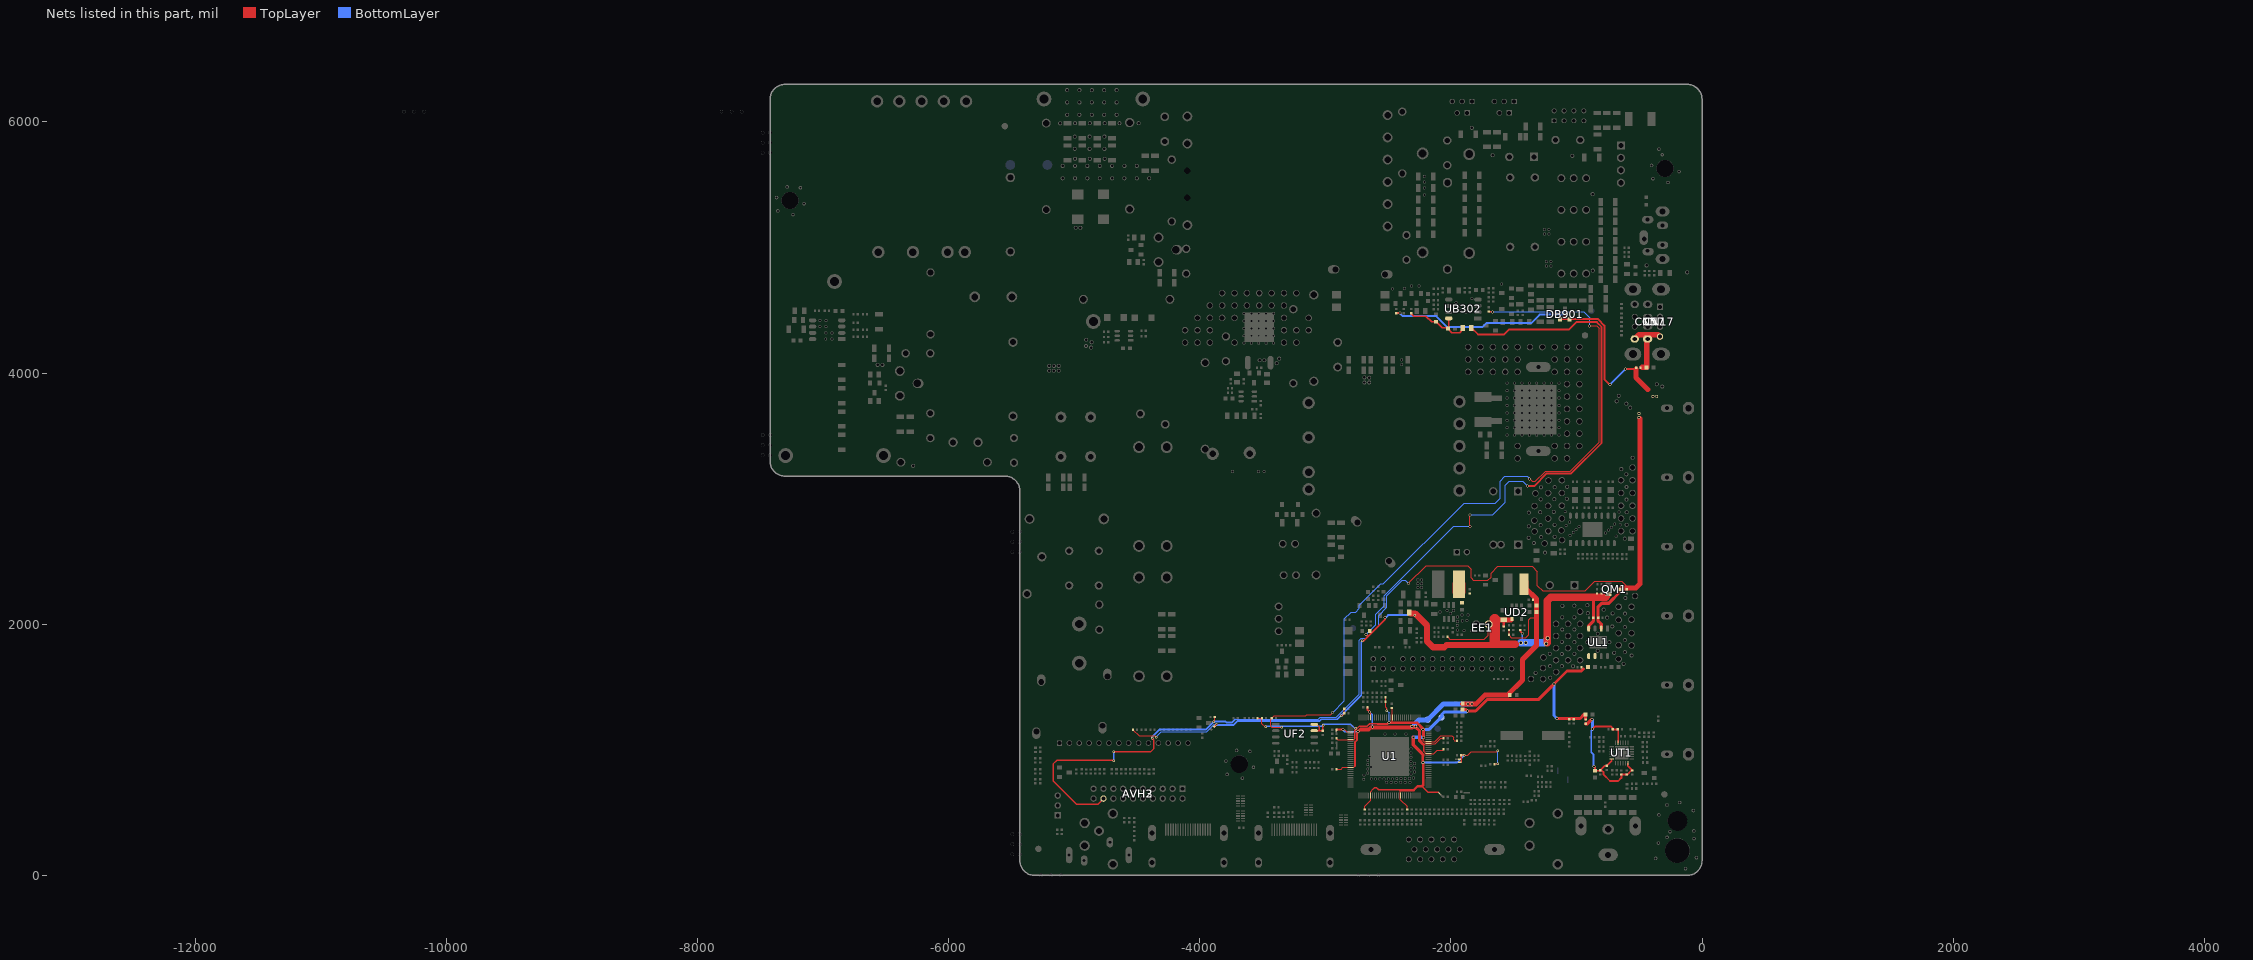
[diagram p0: the nets of this part, all layers, seen from the top]
# Altium PCB MISC84277.PcbDoc (part 6 of 15)
Units mil, origin at the board's own origin, x right, y up, seen from the top; angles counter-clockwise.
Board outline 7422.08 x 6299.21 mil, 2 copper layers (TopLayer, BottomLayer), stack 61.855 mil thick; 709 components, 395 nets, 2812 pads, 811 vias.

## Free pads (board coordinates)
  oval 196.85x157.48 on Keep-Out: 0(-12538.98,6102.21) 0(-375.96,-19.69)
  round 78.74 on Keep-Out: 0(-12170.24,6219.32) 0(-8343.94,6219.32) 0(-4571,-136.8) 0(-744.7,-136.8)
  round 27.56 hole 27.56 unplated: 0(-10337.93,6082.52) 0(-10257.61,6082.52) 0(-10177.3,6082.52) 0(-7809.45,6082.52) 0(-7729.14,6082.52) 0(-7648.82,6082.52) 0(-7481.5,3346.46) 0(-7481.5,3426.77) 0(-7481.5,3507.09) 0(-7481.5,5754.57) 0(-7481.5,5834.89) 0(-7481.5,5915.2) 0(-7422.44,3346.46) 0(-7422.44,3426.77) 0(-7422.44,3507.09) 0(-7422.44,5754.57) 0(-7422.44,5834.89) 0(-7422.44,5915.2) 0(-5492.5,167.48) 0(-5492.5,247.79) 0(-5492.5,328.11) 0(-5492.5,2575.59) 0(-5492.5,2655.9) 0(-5492.5,2736.22) 0(-5433.44,167.48) 0(-5433.44,247.79) 0(-5433.44,328.11) 0(-5433.44,2575.59) 0(-5433.44,2655.9) 0(-5433.44,2736.22) 0(-5266.12,0) 0(-5185.8,0) 0(-5105.49,0) 0(-2737.64,0) 0(-2657.33,0) 0(-2577.01,0)
  round 137.8 on Keep-Out: 0(-5312.1,562.78) 0(-196.85,5708.82)
  round 157.48 on Keep-Out: 0(-197.22,6102.36)
  oval 157.48x196.85 on Keep-Out: 0(-196.85,3503.94)
  round 23.62 hole 15.75 paste-15.75 mask-15.75: VIA5(-7026.5,4370.37) VIA5(-7025.59,4419.29) VIA5(-6979.39,4271.61) VIA5(-6978.49,4320.53) VIA5(-6977.58,4369.46) VIA5(-6976.67,4418.38) VIA5(-6930.47,4270.7) VIA5(-6929.56,4319.62) VIA5(-3740.16,3216.09) VIA5(-3648.83,4297.38) VIA5(-3648.83,4356.44) VIA5(-3648.83,4415.49) VIA5(-3648.83,4474.55) VIA5(-3648.83,4238.33) VIA5(-3589.77,4238.33) VIA5(-3589.77,4297.38) VIA5(-3589.77,4356.44) VIA5(-3589.77,4415.49) VIA5(-3589.77,4474.55) VIA5(-3533.46,3216.09) VIA5(-3530.72,4297.38) VIA5(-3530.72,4474.55) VIA5(-3530.72,4238.33) VIA5(-3530.72,4356.44) VIA5(-3530.72,4415.49) VIA5(-3488.19,3216.54) VIA5(-3471.66,4238.33) VIA5(-3471.66,4297.38) VIA5(-3471.66,4356.44) VIA5(-3471.66,4415.49) VIA5(-3471.66,4474.55) VIA5(-3412.61,4238.33) VIA5(-3412.61,4297.38) VIA5(-3412.61,4356.44) VIA5(-3412.61,4415.49) VIA5(-3412.61,4474.55) VIA5(-2694.55,765.25) VIA5(-2693.4,797.4) VIA5(-2662.7,814) VIA5(-2662.7,847.8) VIA5(-2662.7,881.6) VIA5(-2662.7,915.4) VIA5(-2648.2,948.3) VIA5(-2635.5,864.3) VIA5(-2634.5,769.2) VIA5(-2600.7,769.2) VIA5(-2566.9,769.2) VIA5(-2533.1,769.2) VIA5(-2525.21,1124.32) VIA5(-2513.2,741) VIA5(-2499.3,769.2) VIA5(-2476,741) VIA5(-2466.54,4671.26) VIA5(-2465.5,769.2) VIA5(-2445,1124) VIA5(-2438.8,741) VIA5(-2431.7,770.9) VIA5(-2401.6,741) VIA5(-2397.9,770.9) VIA5(-2392.66,4067.75) VIA5(-2392.66,4105.75) VIA5(-2370.87,4674) VIA5(-2364.4,741) VIA5(-2364.1,770.9) VIA5(-2358.3,1124.32) VIA5(-2330.3,770.9) VIA5(-2327.2,741) VIA5(-2319.2,805.4) VIA5(-2319.2,839.2) VIA5(-2319.2,873) VIA5(-2319.2,906.8) VIA5(-2319.2,940.6) VIA5(-2319.2,974.4) VIA5(-2319.2,1008.2) VIA5(-2314.96,4693.81) VIA5(-2312.19,1186.7) VIA5(-2297.6,775.2) VIA5(-2290.9,823) VIA5(-2290.9,856.8) VIA5(-2290.9,890.6) VIA5(-2281.65,1186.7) VIA5(-2264.25,2293.31) VIA5(-2264.25,2323.31) VIA5(-2264.25,2353.31) VIA5(-2253.94,4693.81) VIA5(-2234.25,2293.31) VIA5(-2234.25,2323.31) VIA5(-2234.25,2353.31) VIA5(-2221.6,898.2) VIA5(-2212.6,5419.29) VIA5(-2212.6,5474.41) VIA5(-2212.6,5521.65) VIA5(-2212.6,5566.93) VIA5(-2087.7,2097.06) VIA5(-2030,2110) VIA5(-2002,2087) VIA5(-1980,2109) VIA5(-1958.5,4561.5) VIA5(-1950,1991) VIA5(-1948.82,1952.76) VIA5(-1948,2022) VIA5(-1948,2058) VIA5(-1929.13,4535.43) VIA5(-1923,4495.5) VIA5(-1912,2074) VIA5(-1910,2027) VIA5(-1895.67,1948.82) VIA5(-1879.92,4487.1) VIA5(-1874,2030) VIA5(-1866,1366) VIA5(-1863,2074) VIA5(-1836.61,1948.82) VIA5(-1834,1366) VIA5(-1832.68,4592.52) VIA5(-1596,4709) VIA5(-1552.98,3506) VIA5(-1552.98,3565.05) VIA5(-1552.98,3624.11) VIA5(-1552.98,3683.16) VIA5(-1552.98,3742.22) VIA5(-1552.98,3801.27) VIA5(-1552.98,3860.33) VIA5(-1552.98,3919.38) VIA5(-1493.92,3506) VIA5(-1493.92,3565.05) VIA5(-1493.92,3624.11) VIA5(-1493.92,3683.16) VIA5(-1493.92,3742.22) VIA5(-1493.92,3801.27) VIA5(-1493.92,3860.33) VIA5(-1493.92,3919.38) VIA5(-1434.87,3506) VIA5(-1434.87,3565.05) VIA5(-1434.87,3624.11) VIA5(-1434.87,3683.16) VIA5(-1434.87,3742.22) VIA5(-1434.87,3801.27) VIA5(-1434.87,3860.33) VIA5(-1434.87,3919.38) VIA5(-1375.81,3506) VIA5(-1375.81,3565.05) VIA5(-1375.81,3624.11) VIA5(-1375.81,3683.16) VIA5(-1375.81,3742.22) VIA5(-1375.81,3801.27) VIA5(-1375.81,3860.33) VIA5(-1375.81,3919.38) VIA5(-1316.76,3742.22) VIA5(-1316.76,3860.33) VIA5(-1316.76,3506) VIA5(-1316.76,3565.05) VIA5(-1316.76,3624.11) VIA5(-1316.76,3683.16) VIA5(-1316.76,3801.27) VIA5(-1316.76,3919.38) VIA5(-1257.7,3565.05) VIA5(-1257.7,3683.16) VIA5(-1257.7,3742.22) VIA5(-1257.7,3801.27) VIA5(-1257.7,3860.33) VIA5(-1257.7,3919.38) VIA5(-1257.7,3506) VIA5(-1257.7,3624.11) VIA5(-1255.91,5108.27) VIA5(-1255.91,5143.7) VIA5(-1240.16,4852.36) VIA5(-1240.16,4887.8) VIA5(-1220.47,5108.27) VIA5(-1220.47,5143.7) VIA5(-1204.72,4852.36) VIA5(-1204.72,4887.8) VIA5(-1198.65,3506) VIA5(-1198.65,3565.05) VIA5(-1198.65,3624.11) VIA5(-1198.65,3683.16) VIA5(-1198.65,3742.22) VIA5(-1198.65,3801.27) VIA5(-1198.65,3860.33) VIA5(-1198.65,3919.38) VIA5(-1139.59,3506) VIA5(-1139.59,3565.05) VIA5(-1139.59,3624.11) VIA5(-1139.59,3683.16) VIA5(-1139.59,3742.22) VIA5(-1139.59,3801.27) VIA5(-1139.59,3860.33) VIA5(-1139.59,3919.38) VIA5(-1090,2896) VIA5(-1082,2786) VIA5(-1054.5,2812.85) VIA5(-1051,2708) VIA5(-1026,2732) VIA5(-1003,2755) VIA5(-979,2778) VIA5(-770,2726) VIA5(-746,2749) VIA5(-722,2772) VIA5(-696,2798) VIA5(-684,2701) VIA5(-660,2894) VIA5(-652,2792) VIA5(-503,3648) VIA5(-503,3678) VIA5(-391.95,3813.95) VIA5(-361.95,3813.95)
  round 31.5 hole 19.68 paste-15.75 mask-15.75: VIA5(-6566,4065) VIA5(-6528,4065) VIA5(-6283.46,3261.81) VIA5(-5200,4018.9) VIA5(-5200,4056.9) VIA5(-5162,4018.9) VIA5(-5162,4056.9) VIA5(-5124,4018.9) VIA5(-5124,4056.9) VIA5(-5112.75,5989.43) VIA5(-5092.52,5551.18) VIA5(-5092.52,5649.61) VIA5(-5057.09,6057.09) VIA5(-5057.09,6155.51) VIA5(-5057.09,6253.94) VIA5(-4996.06,5785.43) VIA5(-4996.06,5883.86) VIA5(-4994.09,5551.18) VIA5(-4994.09,5649.61) VIA5(-4994.09,5706.69) VIA5(-4994.09,5990.16) VIA5(-4988.79,5157.48) VIA5(-4958.66,6057.09) VIA5(-4958.66,6155.51) VIA5(-4958.66,6253.94) VIA5(-4950.79,5157.48) VIA5(-4906.5,4215.9) VIA5(-4905.8,4265.5) VIA5(-4895.67,5551.18) VIA5(-4895.67,5649.61) VIA5(-4877.95,5785.43) VIA5(-4877.95,5883.86) VIA5(-4875.98,5706.69) VIA5(-4875.98,5990.16) VIA5(-4866.6,4203.6) VIA5(-4862.5,4245.5) VIA5(-4860.24,6057.09) VIA5(-4860.24,6155.51) VIA5(-4860.24,6253.94) VIA5(-4797.24,5551.18) VIA5(-4797.24,5649.61) VIA5(-4761.81,6057.09) VIA5(-4761.81,6155.51) VIA5(-4761.81,6253.94) VIA5(-4759.84,5785.43) VIA5(-4759.84,5883.86) VIA5(-4757.87,5990.16) VIA5(-4757.87,5706.69) VIA5(-4698.82,5551.18) VIA5(-4698.82,5649.61) VIA5(-4663.39,6057.09) VIA5(-4663.39,6155.51) VIA5(-4663.39,6253.94) VIA5(-4639.76,5990.16) VIA5(-4600.39,5551.18) VIA5(-4600.39,5649.61) VIA5(-4501.97,5551.18) VIA5(-4501.97,5649.61) VIA5(-4488.19,5990.16) VIA5(-4403.54,5551.18) VIA5(-3524.22,4102.36) VIA5(-3486.22,4102.36) VIA5(-3387.8,4078.74) VIA5(-3368.11,4116.14) VIA5(-2689.57,3925.2) VIA5(-2689.57,3965.17) VIA5(-2651.57,3925.2) VIA5(-2651.57,3963.2) VIA5(-1833.15,5953.3) VIA5(-1668.9,5735.1) VIA5(-1442.5,1851.35) VIA5(-1404.5,1851.35) VIA5(-1381,2687) VIA5(-1380,2780) VIA5(-1379.3,2889) VIA5(-1339,2647) VIA5(-1326,1612) VIA5(-1290,2892.6) VIA5(-1286,2790) VIA5(-1286,2994.6) VIA5(-1283,3090.6) VIA5(-1282,2694) VIA5(-1251,2571) VIA5(-1243,1845) VIA5(-1231,1888) VIA5(-1213,1764) VIA5(-1211,1667) VIA5(-1210,1574) VIA5(-1181,2894) VIA5(-1177,2996) VIA5(-1175,2696) VIA5(-1175,2791) VIA5(-1174,3092) VIA5(-1116,1667) VIA5(-1116,1763) VIA5(-1116,1859) VIA5(-1114,1958) VIA5(-1114,2054.64) VIA5(-1112.2,2145.67) VIA5(-1077,2999) VIA5(-1075,3094) VIA5(-1033.45,5730.08) VIA5(-1028,1665) VIA5(-1017.72,2147.64) VIA5(-1017,1764) VIA5(-1017,1858) VIA5(-1017,1958) VIA5(-1017,2054.64) VIA5(-914.5,1857.5) VIA5(-913.39,2151.57) VIA5(-910,2089) VIA5(-872.05,5425.2) VIA5(-870.08,4816.93) VIA5(-831.5,1788.5) VIA5(-831,1924.5) VIA5(-784,2116) VIA5(-757,2053) VIA5(-738.5,1857) VIA5(-715,1982) VIA5(-713,2086) VIA5(-701,1772) VIA5(-680.5,3775.28) VIA5(-663.82,3818.81) VIA5(-643,3236) VIA5(-625,1684) VIA5(-616,2682) VIA5(-615,1778) VIA5(-615,1874) VIA5(-615,1977) VIA5(-614,2085) VIA5(-611,2209) VIA5(-603,3194) VIA5(-602.2,3756.25) VIA5(-602,2993) VIA5(-602,3093) VIA5(-601,2792) VIA5(-601,2892) VIA5(-572.38,3725.25) VIA5(-562,1751) VIA5(-554,3326) VIA5(-442.4,4857.1) VIA5(-360.13,3911) VIA5(-317.13,3893.19) VIA5(-119,4802)
  round 51.18 hole 39.37 paste-15.75 mask-15.75: VIA5(-4117.27,4243.02) VIA5(-4117.27,4341.45) VIA5(-4018.84,4243.02) VIA5(-4018.84,4341.45) VIA5(-4018.84,4439.88) VIA5(-3920.42,4243.02) VIA5(-3920.42,4341.45) VIA5(-3920.42,4439.87) VIA5(-3920.42,4538.3) VIA5(-3821.99,4439.87) VIA5(-3821.99,4538.3) VIA5(-3821.99,4636.72) VIA5(-3723.57,4243.02) VIA5(-3723.57,4439.87) VIA5(-3723.57,4538.3) VIA5(-3723.57,4636.72) VIA5(-3625.14,4538.3) VIA5(-3625.14,4636.72) VIA5(-3526.72,4538.3) VIA5(-3526.72,4636.72) VIA5(-3428.29,4538.3) VIA5(-3428.29,4636.72) VIA5(-3329.87,4243.02) VIA5(-3329.87,4341.45) VIA5(-3329.87,4439.87) VIA5(-3329.87,4538.3) VIA5(-3329.86,4636.72) VIA5(-3231.44,4243.02) VIA5(-3231.44,4341.45) VIA5(-3231.44,4636.72) VIA5(-3133.02,4341.45) VIA5(-3133.02,4439.87) VIA5(-1862.93,4108.4) VIA5(-1862.93,4206.83) VIA5(-1862.93,4009.98) VIA5(-1764.51,4108.4) VIA5(-1764.51,4206.83) VIA5(-1764.51,4009.98) VIA5(-1666.08,4108.4) VIA5(-1666.08,4206.83) VIA5(-1666.08,4009.98) VIA5(-1567.66,4108.4) VIA5(-1567.66,4206.83) VIA5(-1567.66,4009.98) VIA5(-1469.23,3321) VIA5(-1469.23,4108.4) VIA5(-1469.23,4206.83) VIA5(-1469.23,3419.43) VIA5(-1469.23,4009.98) VIA5(-1370.81,4206.83) VIA5(-1363,1564) VIA5(-1336,2825) VIA5(-1335,2941) VIA5(-1334,2740) VIA5(-1327.5,3042.5) VIA5(-1272.38,4206.83) VIA5(-1267,1651) VIA5(-1266,1563) VIA5(-1264,1736) VIA5(-1254,2644) VIA5(-1226,2841) VIA5(-1226,2942.4) VIA5(-1226,3043.8) VIA5(-1225,2741) VIA5(-1223.2,3145.2) VIA5(-1173.96,3321) VIA5(-1173.96,4108.4) VIA5(-1173.96,4206.83) VIA5(-1173.96,3419.43) VIA5(-1173.96,4009.98) VIA5(-1163,1713.07) VIA5(-1163,1809.72) VIA5(-1163,1906.36) VIA5(-1163,2003) VIA5(-1162,1619) VIA5(-1121,2747) VIA5(-1117,2842.4) VIA5(-1117,2943.8) VIA5(-1117,3045.2) VIA5(-1117,3146.6) VIA5(-1115,2670) VIA5(-1075.53,3321) VIA5(-1075.53,4108.4) VIA5(-1075.53,4206.83) VIA5(-1075.53,3419.43) VIA5(-1075.53,3517.85) VIA5(-1075.53,3616.28) VIA5(-1075.53,3714.7) VIA5(-1075.53,3813.13) VIA5(-1075.53,3911.55) VIA5(-1075.53,4009.98) VIA5(-1067.25,1713.07) VIA5(-1067.25,1809.72) VIA5(-1067.25,1906.36) VIA5(-1067.25,2003) VIA5(-977.11,3419.43) VIA5(-977.11,3517.85) VIA5(-977.11,3616.28) VIA5(-977.11,3714.7) VIA5(-977.11,3813.13) VIA5(-977.11,3911.55) VIA5(-977.11,4009.98) VIA5(-977.11,4108.4) VIA5(-977.11,4206.83) VIA5(-971.5,1713.07) VIA5(-971.5,1809.72) VIA5(-971.5,1906.36) VIA5(-971.5,2003) VIA5(-971.5,2099.64) VIA5(-664,1722) VIA5(-664,1833) VIA5(-664,1929) VIA5(-664,2035) VIA5(-664,2139) VIA5(-645,2741) VIA5(-645,2842.4) VIA5(-645,2943.8) VIA5(-645,3045.2) VIA5(-645,3146.6) VIA5(-562,1831) VIA5(-562,1929) VIA5(-562,2036) VIA5(-562,2139) VIA5(-554,2741) VIA5(-554,2842.4) VIA5(-554,2943.8) VIA5(-554,3045.2) VIA5(-554,3146.6) VIA5(-554,3248) VIA5(-534,2225)

## Via types
v1: diameter 23.62, hole 15.75, TopLayer to BottomLayer, tented both sides, 437 vias
v2: diameter 19.68, hole 11.81, TopLayer to BottomLayer, tented both sides, 353 vias
v3: diameter 31.5, hole 23.62, TopLayer to BottomLayer, tented both sides, 16 vias
v4: diameter 31.5, hole 19.68, TopLayer to BottomLayer, tented both sides, 4 vias
v5: diameter 17.72, hole 9.84, TopLayer to BottomLayer, tented both sides, 1 vias

## Nets (pads, with @x,y where several pads share a name; then routed paths per layer and width w, separated by ;. In a path a pad name is that pad's centre, name@x,y a point inside that pad or via, vN(x,y) a via of type N, cw(c..) or ccw(c..) an arc to the next point about the centre after c; other vN are vias at no path point)
1.15V_STB: 1.15V_STB.1 CD13.1 CD14.2 CD15.2 CD16.2 CF15.1 CF16.2 CF17.2 CF18.2 CF19.2 CF20.2 CF37.1 LD2.2 LF4.JP_2K pad.VIA5@-1834,1366 pad.VIA5@-1866,1366 pad.VIA5@-2281.65,1186.7 pad.VIA5@-2312.19,1186.7 RD6.2 U1.50 U1.55 U1.90 U1.100 U1.118 | length 4346.5
  TopLayer w8: CF18.2@-2912.27,846 -2874,846 -2859.94,860.06 U1.118@-2800.46,860.06 ; -2847,1160 -2830.53,1143.53 U1.100@-2800.46,1143.53 ; -2834.94,860.06 U1.118@-2800.46,860.06 ; -2764.34,868.98 -2773.25,860.06 U1.118@-2800.46,860.06 ; v1@-2650,1299 -2639.05,1288.05 U1.90@-2639.05,1257.7 ; -2220,1042.57 -2213.54,1049.04 U1.55@-2178.42,1049.04 -2143,1049.04 ; -2217.01,986.64 -2200.67,970.3 U1.50@-2178.42,970.3 -2135.9,970.3 -2107.91,998.29 -2066.17,998.29 CF20.2@-2058.46,1006 ; -2133.8,1049.04 -2143,1049.04 ; CF19.2@-2058.73,1092 -2082.08,1092 -2125.05,1049.04 -2143,1049.04 ; RD6.2@-1536.73,1954 -1536.73,1910.73 -1519,1893 -1404,1893 -1380,1917 -1380,2036 -1366,2050 -1320.89,2050 -1318.89,2048
  TopLayer w15: CF16.2@-2912.27,1161 v1@-2868.47,1161 ; -2764.34,868.98 -2764.34,1061.98 -2747.34,1078.98 -2747.34,1133.66 v1@-2737,1144 ; CF17.2@-2665.27,1337 -2665.27,1320.47 v1@-2646.9,1302.1 ; -2220,1042.57 -2216.5,1039.07 -2216.5,991.07
  TopLayer w24: v1@-2740.83,1144.13 -2722.47,1162.5 -2718.5,1162.5 -2701.4,1162.5
  TopLayer w25: pad.VIA5@-2311.02,1178.5 -2307.49,1178.5 -2306.36,1179.63 -2280.03,1179.63 -2250,1149.61 -2250,1072.57 -2220,1042.57
  TopLayer w30: -2718.5,1162.5 -2655.38,1162.5 -2639.38,1178.5 pad.VIA5@-2311.02,1178.5
  TopLayer w40: CF15.1@-1906.19,1366 pad.VIA5@-1866,1366 pad.VIA5@-1834,1366 -1799.28,1366 -1728.02,1437.26 -1547.74,1437.26 -1430.76,1554.24 -1430.76,1719.24 -1318.89,1831.11 -1318.89,2048 -1318.89,2200.89 -1404,2286 LD2.2@-1404,2339
  BottomLayer w12: v1(-2648,1301) -2626,1279 v1@-2626,1181.4
  BottomLayer w15: v1(-2860,1160) -2844,1144 v1(-2740.7,1144)
  BottomLayer w40: -2291.34,1200.79 -2254.97,1237.16 -2187.84,1237.16 1.15V_STB.1@-2185,1240 -2059,1366 pad.VIA5@-1866,1366 pad.VIA5@-1834,1366
  other v1: -2625.9,1181.4
3V3_STB: 3V3_STB.1 CF2.2 CF5.1 CF6.2 CF7.2 CF8.2 CF9.2 CF10.2 CF11.2 CL3.1 CL4.1 CT2.1 LF1.JP_2K LF2.JP_2K LF3.JP_2K pad.VIA5@-2221.6,898.2 RB354.2 RF2.2 RF3.2 RK4.2 RK18.2 RM3.1 RT3.1 RT4.1 RT7.1 RT18.1 U1.7 U1.22 U1.56 U1.79 U1.104 UF2.7 UF2.8 UL1.5 UL1.6 | length 12982.8
  TopLayer w8: RK4.2@-3540.27,1251 RF2.2@-3505.73,1251 -3505.73,1209.03 -3480.4,1183.7 v2(-3475.7,1183.7) ; v2(-3348.3,1180.4) -3429,1180.4 -3434.6,1186 -3434.6,1244.13 RF3.2@-3427.73,1251 -3408.89,1269.84 -3155.13,1269.84 -3146.97,1278 -2958.22,1278 -2942.91,1293.31 v1(-2942.91,1295.27) ; CF8.2@-2912.27,1091 -2901.8,1080.53 -2866,1080.53 ; -2895.53,1080.53 -2866,1080.53 ; -2765.84,1086.64 -2771.95,1080.53 U1.104@-2800.46,1080.53 -2866,1080.53 ; CF11.2@-2688,524.73 -2688,549.35 -2639.05,598.31 U1.7@-2639.05,635.65 -2639.05,666.95 -2618,688 ; RM3.1@-2520.27,1417 -2520.27,1340.27 -2511,1331 v2@-2511,1313 ; CF6.2@-2466.5,1333 -2465.82,1332.32 U1.79@-2465.82,1257.7 -2465.82,1215.04 ; -2402.83,677.83 U1.22@-2402.83,635.65 -2402.83,602.83 -2350,550 CF7.2@-2350,524.73 ; -2220,1080.8 -2220,1072.98 -2211.81,1064.79 U1.56@-2178.42,1064.79 -2127.68,1064.79 -2079.47,1113 -2022,1113 -2021.84,1112.84 -1992.2,1112.84 -1979.31,1099.96 -1979.31,1078.31 -1972,1071 CF10.2@-1951.73,1071 CF10.2@-1951.73,1072.38 ; v2(-1893,958) -1866.07,958 -1838.57,985.5 v2@-1634.5,985.5 ; RT18.1@-1653.27,883 -1648.27,888 v2(-1628,888) ; v1(-1372.7,3157.3) -1353.6,3138.2 -1327.7,3138.2 -1245.61,3220.29 -1051.37,3220.29 -820.68,3450.97 -820.68,4356.3 -840.37,4375.98 v1(-895.67,4375.98)
  TopLayer w11.81: RB354.2@-1700,4490.27 v1@-1672.77,4490.27
  TopLayer w12: UF2.8@-3091.46,1203 UF2.8@-3088.46,1203 ; UF2.7@-3088.46,1153 -3050,1153 ; UF2.8@-3067,1202 -3050,1185 -3050,1153 ; v2@-3020,1194 -3020,1155.73 -3022.73,1153 -3050,1153 ; -2765.84,1086.64 -2765.84,1151.93 -2729.27,1188.5 -2666.14,1188.5 -2647.14,1207.5 -2586.9,1207.5 ; -2618,688 -2609.16,696.84 -2590.37,696.84 -2574.8,681.27 -2406.27,681.27 -2402.83,677.83 ; -2231.21,709.79 -2181.45,660.03 LF2.JP_2K@-2095.63,660.03 ; -2220,1080.8 v1(-2220,1099.6) ; CF9.2@-1918.27,958 v2@-1893,958
  TopLayer w15: -2586.9,1206 -2506.5,1206 v1@-2494.62,1217.88 ; LF3.JP_2K@-1918.27,903 CF9.2@-1918.27,958
  TopLayer w20: v1@-2491,1214.22 -2269.51,1214.22 -2240.24,1184.95 ; -2402.83,677.83 -2297,677.83 -2265.03,709.79 -2231.21,709.79 -2221.6,719.4 pad.VIA5@-2221.6,898.2 ; pad.VIA5@-2223.5,898.2 -2223.5,951.64
  TopLayer w25: v1(-2300,1099.7) -2300,1039.55 -2241.5,981.05 -2241.5,980.72 -2223.5,962.72 -2223.5,951.64 ; -2240.24,1184.95 v1@-2220,1164.71 ; v1(-2220,1099.6) v1@-2220,1162.7 ; CF5.1@-1907.19,1321 -1880,1321 ; v1(-1868,1309) -1803.25,1309 -1712.49,1399.76 -1303.84,1399.76 -1076.26,1627.34 -961.04,1627.34 -945.23,1643.15 ; v1@-1154,1248.76 -971.64,1248.76 CT2.1@-938.2,1282.2 ; RT7.1@-928.4,1245.83 -928.4,1278.9 -929.06,1279.56 CT2.1@-928.4,1280.21
  BottomLayer w8: v1(-2942.91,1295.27) -2848.43,1389.76 -2848.43,2043.31 -2795.28,2096.46 -2759.84,2096.46 -2730.32,2125.98 -2730.32,2151.57 -2559.06,2322.83 -2537.64,2322.83 -1895.48,2965 -1648.4,2965 -1608.4,3005 -1608.4,3140.5 -1571.3,3177.6 -1393,3177.6 v1(-1372.7,3157.3) ; v2(-2510,1312) -2493,1295 v1(-2493,1216.27) ; v1@-1669,4487 -940.94,4487 -895.67,4441.73 v1(-895.67,4375.98) ; v2(-1628,888) v2(-1628,992)
  BottomLayer w12: v2@-3475.44,1188 -3032.01,1188 -3017.01,1203 -2799.05,1203 v2@-2761.05,1165 ; pad.VIA5@-2222.16,898.84 -1950.16,898.84 -1893,956 v2(-1893,958)
  BottomLayer w25: v1(-2300,1099.7) v1@-2220,1099.7 ; v1(-2221.6,1162.7) -2173.5,1162.7 3V3_STB.1@-2077.6,1258.6 ; 3V3_STB.1@-2072.5,1263.7 -2072.5,1281.5 -2053,1301 v1@-1876,1301 ; v1(-1179.34,1524.34) -1179.34,1273.34 v1(-1154,1248)
  other v1: -1669.5,4487
  other v2: -2759.3,1170 -3018,1196
3V3_TUN: CT5.2 CT6.1 CT9.1 CT18.2 CT27.1 CT30.2 LT1.1 LT2.2 RT7.2 UT1.11 UT1.18 UT1.24 | length 1397.3
  TopLayer w8: -720.63,916.63 UT1.18@-720.63,926.1
  TopLayer w10: CT27.1@-672.13,1162.47 -669.45,1159.79 UT1.11@-669.45,1056.02 ; UT1.24@-590.71,894.6 -590.71,872 -585.12,866.41
  TopLayer w14: CT5.2@-814.06,833.2 -796.94,833.2 -784.25,820.51 -784.25,802.51 -733.15,751.41 -667.41,751.41 -642.74,776.08 LT2.2@-642.74,802.68 LT1.1@-600.14,802.69 -595.54,802.69 -562.08,836.15 -554.86,836.15 -585.12,866.41 ; CT18.2@-759.1,873.9 -720.24,912.76
  TopLayer w15: v1(-874,1164) -851,1187 -726,1187 -712.27,1173.27 CT30.2@-712.27,1163 -672.66,1163 CT27.1@-672.13,1162.47 ; v1(-862,867.76) -851.63,857.39 CT6.1@-851.63,833.2 -814.06,833.2 CT5.2@-809.65,837.61 ; CT5.2@-809.75,837.72 -774.75,872.72 -771,872.72
  TopLayer w25: RT7.2@-928.4,1207.67 -913.95,1207.67 -881.52,1240.1 v1@-875.4,1240.1
  BottomLayer w15: v1@-882.34,1155.66 -882.34,981.93 -865.31,964.9 v1@-865.31,871.07
  BottomLayer w25: v1(-874,1164) v1@-874,1240.1
  other v1: -875.43,1240.1
5V_M: AVH2.18 AVH3.18 CL42.1 CM2.1 DB901.1 DB901.3 F2.1 pad.VIA5@-361.95,3813.95 pad.VIA5@-391.95,3813.95 pad.VIA5@-503,3648 pad.VIA5@-503,3678 QM1.D RB346.1 RK2.2 UL1.2 | length 11495.5
  TopLayer w8: -3880.77,1230.94 RK2.2@-3880.77,1261.1 RK2.2@-3875.69,1261.1 ; v1(-2338.58,2324.8) -2198.77,2464.62 -1865.62,2464.62 -1840,2439 -1840,2369 -1821,2350 -1706,2350 -1681,2375 -1681,2408 -1629,2460 -1352.75,2460 -1311.02,2418.28 -1311.02,2306.34 -1270.43,2265.75 -930.58,2265.75 -854.33,2342 -639,2342 -601,2304 CM2.1@-601,2278.73
  TopLayer w12: AVH2.18@-4767.74,610.96 -4813.74,564.96 -4980.69,564.96 -5168.5,752.77 -5168.5,886.33 -5139.99,914.84 -4687.64,914.84 v2(-4683.8,911) ; v2(-4683.8,985.7) -4596.5,985.7 ; -4645.7,985.7 -4596.5,985.7 ; v2(-4379.74,1092.26) -4368.1,1080.62 -4368.1,1006.8 -4389.2,985.7 -4596.5,985.7
  TopLayer w15.75: RB346.1@-2435,4476.77 -2407.23,4476.77 v1(-2407,4477) ; DB901.1@-1131,4429 -1096,4429 ; v1(-1093,4465.5) -1093,4432 -1096,4429 ; v1(-734.25,3907.47) -777.56,3950.78 -777.56,4377.95 -828.61,4429 DB901.3@-1056,4429 -1096,4429 ; v1(-608.27,4033.46) -530.58,4033.46 -528.13,4031
  TopLayer w25: UL1.2@-803,1965.55 -803,2002 -830,2029 -830,2136 -798.5,2167.5 -742.5,2167.5 -653.72,2256.28 QM1.D@-653.72,2278
  TopLayer w40: QM1.D@-641.72,2290 -527,2290 -496,2321 -496,3637 ; -528.13,4031 -528.13,3964.19 -432.72,3868.78
  BottomLayer w8: -3715.39,1245 -3055.62,1245 -3040.62,1260 -2912.65,1260 -2731,1441.65 -2731,1870.55 -2714.16,1887.39 -2675.61,1887.39 -2576.77,1986.22 -2576.77,2068.9 -2509.84,2135.83 -2509.84,2225.75 -2387.17,2348.43 -2362.2,2348.43 v1(-2338.58,2324.8)
  BottomLayer w12: v2(-4683.8,911) v2(-4683.8,985.7)
  BottomLayer w15: v2(-4379.74,1092.26) -4379.74,1102.32 -4321.89,1160.17 -3951.68,1160.17 v2@-3888.34,1223.51 ; v2(-3888.2,1223.51) -3887.11,1224.6 -3793.15,1224.6 -3786.15,1217.6 -3742.8,1217.6 -3718.9,1241.5
  BottomLayer w15.75: v1(-2407,4477) -2383.5,4453.5 -2116.5,4453.5 -2029.5,4366.5 -1750,4366.5 -1718,4398.5 -1360.5,4398.5 -1293.5,4465.5 v1(-1093,4465.5) ; v1(-734.25,3907.47) v1(-608.27,4033.46)
5V_P: CB302.2 RB301.1 RB350.2 RB356.2 UB302.8 | length 575
  TopLayer w11.81: RB356.2@-2319.5,4476.77 -2318.77,4476.77 -2294.5,4452.5 -2199,4452.5 -2154.5,4408 -2119.5,4408 RB350.2@-2119.5,4407.72 -2115.72,4407.72 -2070.18,4362.18 -2022.15,4362.18 -2017.56,4366.77 -2017.56,4396.03 UB302.8@-2017.56,4436 ; CB302.2@-2022.31,4354.5 -2022.31,4352.81 -1992,4322.5 -1931,4322.5 -1905.09,4348.41 RB301.1@-1905.09,4360.5
5V_STB: 5V_STB.1 CD3.1 CD4.2 CD11.2 CD12.1 CL2.2 CM1.1 EE1.1 LD12.2 pad.VIA5@-1231,1888 pad.VIA5@-1243,1845 pad.VIA5@-1404.5,1851.35 pad.VIA5@-1442.5,1851.35 QM1.S R5V.1 RB301.2 RB384.1 RD8.1 RD12.2 RF8.2 RF9.2 RK1.1 RK15.1 RM1.2 UD2.4 UL1.4 | length 11238.4
  TopLayer w8: RK15.1@-4532.83,1160 -4483.93,1111.1 -4406.5,1111.1 ; -4387.54,1111.1 -4406.5,1111.1 ; v2@-4349.86,1101.43 -4359.53,1111.1 -4406.5,1111.1 ; v2(-2873,1273) -2867.73,1273 RF8.2@-2849.73,1291 RF9.2@-2849.73,1327 ; RD12.2@-2027.27,1900 -2008.07,1880.8 -1733.89,1880.8 -1702.54,1912.16 -1702.54,2007.77 EE1.1@-1704.22,2009.45
  TopLayer w9.84: v1(-1848.43,2779.53) v1(-1848.43,2871.4)
  TopLayer w10: RD8.1@-1447.73,1954 -1447.73,1943.51 v1(-1431.03,1926.81)
  TopLayer w11.81: RB384.1@-2653.54,1944.88 RB384.1@-2645.5,1944.88
  TopLayer w15: RK1.1@-3885.25,1185.39 -3868.38,1202.26 v2(-3867.19,1202.26) ; v2(-2705,1867) -2695.99,1867 -2659.45,1903.54 ; v1(-2677.16,1917.32) -2663.38,1903.54 -2659.45,1903.54 ; v1(-2523.62,2055.11) -2523.62,2039.38 -2659.45,1903.54 ; RB301.2@-1836.91,4360.5 -1784.66,4308.25 -1576.25,4308.25 -1535.93,4348.57 -1058.91,4348.57 -1001.85,4405.63 -838.45,4405.63 -801.18,4368.36 -801.18,3442.9 -1043.29,3200.79 -1236.21,3200.79 -1336.6,3100.4 v1(-1389,3100.4)
  TopLayer w17: CD12.1@-1580,1982.73 CD11.2@-1580,2023 ; CD11.2@-1578.16,2033 CD11.2@-1576,2030.84
  TopLayer w25: UL1.4@-903,1965.55 -903,1988 -866,2025 -866,2203.33 -854.33,2215
  TopLayer w40: -1622,2040.95 -1614.05,2033 -1578.16,2033 -1523.04,2033 UD2.4@-1522.53,2032.49
  TopLayer w50: R5V.1@-2324,2089 -2321,2086 -2286.38,2086 -2191,1990.62 -2191,1864 -2143,1816 -2052.4,1816 -2034.59,1833.8 -1673.01,1833.8
  TopLayer w60: -1668.01,1838.8 -1490,1838.8 ; pad.VIA5@-1233,1851 -1233,2186.29 -1204.29,2215 -854.33,2215 -768,2215 QM1.S@-758,2225
  TopLayer w85: -1650.34,1856.48 -1650.34,2040.95
  TopLayer w100: LD12.2@-1935.83,2258.24 LD12.2@-1935.83,2318.35 LD12.2@-1935.83,2259.82
  BottomLayer w8: v2@-4349.86,1101.43 -4307.62,1143.67 -3944.84,1143.67 -3886.26,1202.26 v2(-3867.19,1202.26) ; v2(-2873,1273) v2@-2870,1273
  BottomLayer w9.84: v1(-2677.16,1917.32) -2598.5,1995.98 -2598.5,2079.33 -2531.17,2146.66 -2531.17,2226.89 -1978.54,2779.53 v1(-1848.43,2779.53) ; v1(-1848.43,2871.4) -1667.8,2871.4 -1568.1,2971.1 -1568.1,3108.4 -1537.3,3139.2 -1427.4,3139.2 v1@-1388.6,3100.4
  BottomLayer w10: v1(-1431.03,1926.81) -1431.19,1926.81 -1431.19,1853.93 pad.VIA5@-1428.6,1851.35
  BottomLayer w15: v2(-3867.19,1202.26) -3861.13,1196.2 -3734.32,1196.2 -3702.02,1228.5 -3048.78,1228.5 -3033.78,1243.5 -2905.81,1243.5 -2714.5,1434.81 -2714.5,1857.5 v2(-2705,1867) ; v1(-2523.62,2055.11) -2516.89,2055.11 -2500,2072 -2284,2072 -2285,2071 v2(-2287,2071)
  BottomLayer w60: pad.VIA5@-1442.5,1851.35 -1428.6,1851.35 -1255.65,1851.35 pad.VIA5@-1232,1875
  other v2: -4348.4,1101.7
5V_USB: CN5.1 CN5.5 CN7.1@-433.46,4271.65 CN17.4 CU1.2 F2.2 | length 474.3
  TopLayer w45: CN5.1@-536.61,4271.65 -501.77,4306.5 -351.09,4306.5 CN17.4@-335.48,4290.89 ; -476.63,4045.5 CU1.2@-441.81,4045.5 ; CU1.2@-442,4045.69 CN7.1@-442,4263.12